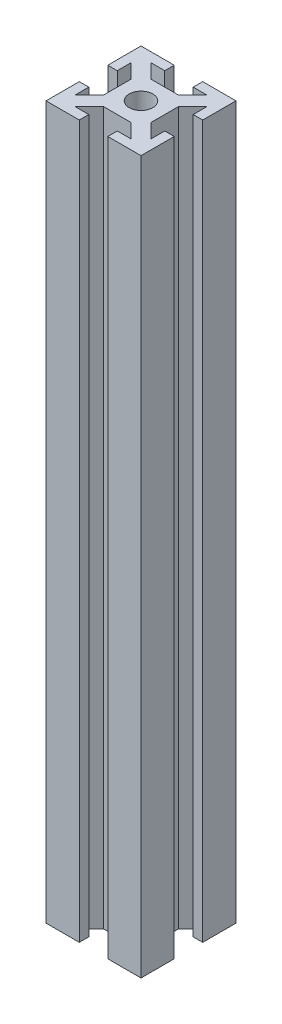
SolidWorks part; units mm, degrees
ref_plane "Front Plane" through (0, 0, 0) normal (0, 0, 1) x (1, 0, 0)
ref_plane "Top Plane" through (0, 0, 0) normal (0, 1, 0) x (1, 0, 0)
ref_plane "Right Plane" through (0, 0, 0) normal (1, 0, 0) x (0, 0, -1)
other "Configuration Table"
sketch "Sketch1" plane through (0, 0, 0) normal (0, 1, 0) x (1, 0, 0)
  line L0 (-6, 20) -> (-6, 16)
  line L5 (-20, 20) -> (-6, 20)
  line L6 (-20, 20) -> (-20, 6)
  line L7 (-20, -20) -> (-6, -20)
  line L8 (20, 20) -> (20, 6)
  line L9 (-20, 20) -> (20, -20) construction
  line L10 (-20, -20) -> (20, 20) construction
  line L11 (-6, 16) -> (-11.7574, 16)
  line L12 (-11.7574, 16) -> (-5.7574, 10)
  line L13 (5.7574, 10) -> (11.7574, 16)
  line L14 (11.7574, 16) -> (6, 16)
  line L15 (6, 16) -> (6, 20)
  line L16 (20, 6) -> (16, 6)
  line L17 (16, 6) -> (16, 11.7574)
  line L18 (16, 11.7574) -> (10, 5.7574)
  line L19 (10, -5.7574) -> (16, -11.7574)
  line L20 (16, -11.7574) -> (16, -6)
  line L21 (16, -6) -> (20, -6)
  line L22 (6, -20) -> (6, -16)
  line L23 (6, -16) -> (11.7574, -16)
  line L24 (11.7574, -16) -> (5.7574, -10)
  line L25 (-5.7574, -10) -> (-11.7574, -16)
  line L26 (-11.7574, -16) -> (-6, -16)
  line L27 (-6, -16) -> (-6, -20)
  line L28 (-20, -6) -> (-16, -6)
  line L29 (-16, -6) -> (-16, -11.7574)
  line L30 (-16, -11.7574) -> (-10, -5.7574)
  line L31 (-10, 5.7574) -> (-16, 11.7574)
  line L32 (-16, 11.7574) -> (-16, 6)
  line L33 (-16, 6) -> (-20, 6)
  line L34 (6, 20) -> (20, 20)
  line L35 (-20, -6) -> (-20, -20)
  line L36 (20, -6) -> (20, -20)
  line L37 (6, -20) -> (20, -20)
  line L39 (-5.7574, -10) -> (5.7574, -10)
  line L40 (-10, -5.7574) -> (-10, 5.7574)
  line L41 (-5.7574, 10) -> (5.7574, 10)
  line L42 (10, -5.7574) -> (10, 5.7574)
  line L43 (-10, -10) -> (10, 10) construction
  line L44 (-10, 10) -> (10, -10) construction
  circle A0 centre (0, 0) radius 5
  point P0 (0, 0)
  point P5 (0, 0)
  point P37 (0, 0)
  dimension "D10" = 10
  dimension "D1" = 40
  dimension "D2" = 4
  dimension "D3" = 4
  dimension "D4" = 14
  dimension "D5" = 14
  dimension "D6" = 3
  dimension "D7" = 3
  dimension "D8" = 4
  dimension "D9" = 20
extrude "Boss-Extrude1" add sketch "Sketch1" along normal blind 300
